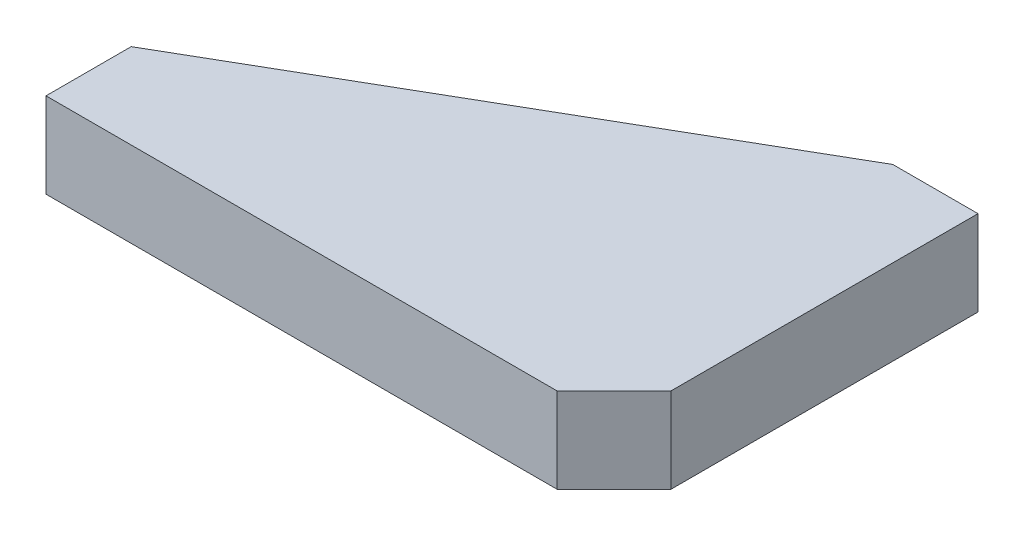
SolidWorks part; units mm, degrees
ref_plane "前视基准面" through (0, 0, 0) normal (0, 0, 1) x (1, 0, 0)
ref_plane "上视基准面" through (0, 0, 0) normal (0, 1, 0) x (1, 0, 0)
ref_plane "右视基准面" through (0, 0, 0) normal (1, 0, 0) x (0, 0, -1)
sketch "草图1" plane through (0, 0, 0) normal (0, 1, 0) x (1, 0, 0)
  line L0 (0, 0) -> (-30, 0)
  line L1 (-30, 0) -> (-200, -98.1495)
  line L2 (-200, -98.1495) -> (-200, -128.1495)
  line L3 (-200, -128.1495) -> (-20, -128.1495)
  line L4 (-20, -128.1495) -> (0, -108.1495)
  line L5 (0, -108.1495) -> (0, 0)
  dimension "D1" = 30
  dimension "D2" = 30
  dimension "D3" = 30
  dimension "D4" = 200
  dimension "D5" = 45
  dimension "D6" = 20
extrude "凸台-拉伸1" add sketch "草图1" along normal blind 30
